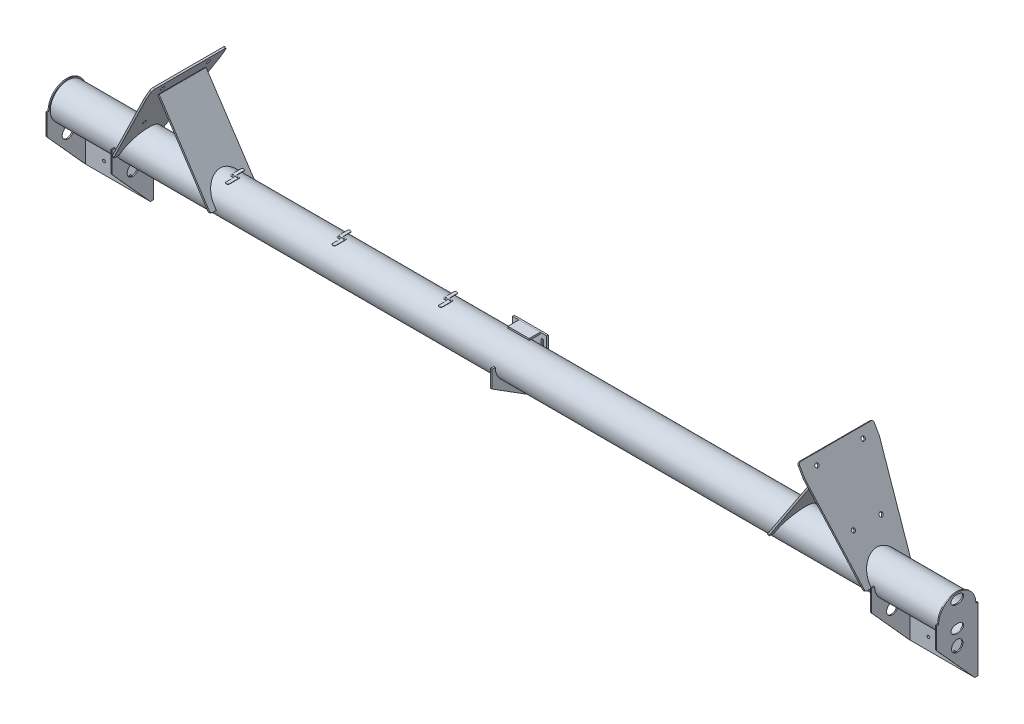
from build123d import *

# Parameters (mm, degrees)
SKETCH1_R             = 82.5
SKETCH1_R_2           = 79.5
BOSS_EXTRUDE1_DEPTH   = 2085
SKETCH2_R             = 26.5
SKETCH2_RX            = 30
SKETCH2_RY            = 20
BOSS_EXTRUDE2_DEPTH   = 5
SKETCH3_R             = 26.5
BOSS_EXTRUDE3_DEPTH   = 5
SKETCH4_W             = 300
SKETCH4_H             = 300
BOSS_EXTRUDE4_DEPTH   = 8
EXTRUDE_THIN1_DEPTH   = 175
EXTRUDE_THIN2_DEPTH   = 110
CUT_EXTRUDE1_DEPTH    = 600
SKETCH19_R            = 9
CUT_EXTRUDE5_DEPTH    = 8
FILLET1_R             = 10
FILLET2_R             = 10
SKETCH7_W             = 160
SKETCH7_H             = 268
BOSS_EXTRUDE5_DEPTH   = 8
BOSS_EXTRUDE6_DEPTH   = 4
SKETCH9_W             = 100
SKETCH9_H             = 52
BOSS_EXTRUDE7_DEPTH   = 8
FILLET3_R             = 10
CUT_EXTRUDE2_DEPTH    = 8
SKETCH17_R            = 6.5
CUT_EXTRUDE3_DEPTH    = 8
SKETCH18_R            = 6.5
CUT_EXTRUDE4_DEPTH    = 8
CUT_EXTRUDE6_DEPTH    = 8
CUT_EXTRUDE7_DEPTH    = 8
BOSS_EXTRUDE8_START   = 82.5
SKETCH22_R            = 3
BOSS_EXTRUDE8_DEPTH   = 1.5
BOSS_EXTRUDE8_2_DEPTH = 1.5
BOSS_EXTRUDE8_3_DEPTH = 1.5


with BuildPart() as part:
    # Sketch1 → Boss-Extrude1 (new, symmetric)
    with BuildSketch(Plane(origin=(0, 0, 0), x_dir=(0, 0, -1), z_dir=(1, 0, 0))):
        Circle(SKETCH1_R)
        Circle(SKETCH1_R_2, mode=Mode.SUBTRACT)
    extrude(amount=BOSS_EXTRUDE1_DEPTH, both=True)


with BuildPart() as body_2:
    # Sketch2 → Boss-Extrude2 (new body)
    with BuildSketch(Plane(origin=(2085, 0, 0), x_dir=(0, 0, -1), z_dir=(1, 0, 0))):
        with BuildLine():
            Line((87.5, 0), (97.5, 0))
            Line((97.5, 0), (97.5, -300))
            Line((97.5, -300), (82.5, -300))
            Line((82.5, -300), (-97.5, -100))
            Line((-97.5, -100), (-97.5, 0))
            Line((-97.5, 0), (-87.5, 0))
            ThreePointArc((-87.5, 0), (0, 87.5), (87.5, 0))
        make_face()
        with Locations((0, -130)):
            Circle(SKETCH2_R, mode=Mode.SUBTRACT)
        with Locations((0, 59.5)):
            Ellipse(SKETCH2_RX, SKETCH2_RY, mode=Mode.SUBTRACT)
        with Locations((0, -59.5)):
            Ellipse(SKETCH2_RX, SKETCH2_RY, mode=Mode.SUBTRACT)
    extrude(amount=BOSS_EXTRUDE2_DEPTH)


with BuildPart() as body_3:
    # Sketch3 → Boss-Extrude3 (new body)
    with BuildSketch(Plane.ZY.offset(-1785)):
        with BuildLine():
            Line((97.5, 0), (97.5, -100))
            Line((97.5, -100), (-82.5, -300))
            Line((-82.5, -300), (-97.5, -300))
            Line((-97.5, -300), (-97.5, 0))
            Line((-97.5, 0), (-82.6, 0))
            ThreePointArc((-82.6, 0), (0, -82.6), (82.6, 0))
            Line((82.6, 0), (97.5, 0))
        make_face()
        with Locations((0, -130)):
            Circle(SKETCH3_R, mode=Mode.SUBTRACT)
    extrude(amount=BOSS_EXTRUDE3_DEPTH)


with BuildPart() as body_4:
    # Sketch4 → Boss-Extrude4 (new body)
    with BuildSketch(Plane(origin=(0, 0, -82.6), x_dir=(-1, 0, 0), z_dir=(0, 0, -1))):
        with Locations((-1935, -150)):
            Rectangle(SKETCH4_W, SKETCH4_H)
    extrude(amount=BOSS_EXTRUDE4_DEPTH)


with BuildPart() as body_5:
    # Sketch 5_3 → Extrude-Thin1 (new, symmetric)
    with BuildSketch(Plane.XY):
        Polygon((1513.109525527, 413.651394229), (1762, -20), (1768.938422308, -16.017752408), (1520.047947835, 417.633641821), align=None)
    extrude(amount=EXTRUDE_THIN1_DEPTH, both=True)


with BuildPart() as body_6:
    # Sketch 5_3 2 → Extrude-Thin2 (new, symmetric)
    with BuildSketch(Plane.XY):
        Polygon((1552.932001443, 344.267171152), (1312, -20), (1305.327470607, -15.58668475), (1546.259472049, 348.680486402), align=None)
    extrude(amount=EXTRUDE_THIN2_DEPTH, both=True)


with BuildPart() as cut_extrude1_tool:
    # Sketch6 → Cut-Extrude1 (new body)
    with BuildSketch(Plane.ZY.offset(-1785)):
        with BuildLine():
            Line((-82.5, 0), (-82.5, -100))
            Line((-82.5, -100), (82.5, -100))
            Line((82.5, -100), (82.5, 0))
            ThreePointArc((82.5, 0), (0, 82.5), (-82.5, 0))
        make_face()
    extrude(amount=CUT_EXTRUDE1_DEPTH)


with BuildPart() as body_6_1:
    add(body_6.part)

    # Cut-Extrude1: cut by cut_extrude1_tool
    add(cut_extrude1_tool.part, mode=Mode.SUBTRACT)

    # Fillet2
    fillet2_edges = [body_6_1.edges().sort_by_distance(p)[0] for p in [
        (1308.663735303, -17.793342375, -110),
        (1308.663735303, -17.793342375, 110),
    ]]
    fillet(fillet2_edges, radius=FILLET2_R)


with BuildPart() as body_5_1:
    add(body_5.part)

    # Cut-Extrude1: cut by cut_extrude1_tool
    add(cut_extrude1_tool.part, mode=Mode.SUBTRACT)

    # Sketch19 → Cut-Extrude5 (cut)
    with BuildSketch(Plane(origin=(1323.705177746, 759.729160648, 0), x_dir=(0, 0, -1), z_dir=(0.8673027884579109, 0.4977809489455502, 0))):
        with Locations(Location((-108.807238687, -434.436087811, 0), (0, 0, 90))):
            Circle(SKETCH19_R)
        with Locations(Location((-65, -690.718989774, 0), (0, 0, 90))):
            Circle(SKETCH19_R)
        with Locations(Location((65, -690.718989774, 0), (0, 0, 90))):
            Circle(SKETCH19_R)
        with Locations(Location((108.807238687, -434.436087811, 0), (0, 0, 90))):
            Circle(SKETCH19_R)
        Polygon((-175, -454.436087811), (-175, -894.436087811), (-110, -894.436087811), align=None)
        Polygon((110, -894.436087811), (175, -454.436087811), (175, -894.436087811), align=None)
    extrude(amount=-CUT_EXTRUDE5_DEPTH, mode=Mode.SUBTRACT)

    # Fillet1
    fillet1_edges = [body_5_1.edges().sort_by_distance(p)[0] for p in [
        (1516.578736681, 415.642518025, 175),
        (1516.578736681, 415.642518025, -175),
        (1765.469211154, -18.008876204, -110),
        (1765.469211154, -18.008876204, 110),
    ]]
    fillet(fillet1_edges, radius=FILLET1_R)


with BuildPart() as body_7:
    # Mirror2: mirrored copy
    add(body_2.part.mirror(Plane(origin=(0, 0, 0), x_dir=(0, 0, 1), z_dir=(1, 0, 0))))


with BuildPart() as body_8:
    # Mirror2 2: mirrored copy
    add(body_4.part.mirror(Plane(origin=(0, 0, 0), x_dir=(0, 0, 1), z_dir=(1, 0, 0))))

    # Sketch18 → Cut-Extrude4 (cut)
    with BuildSketch(Plane.XY.offset(-82.6)):
        with Locations((-1873.483275722, -118.336372909)):
            Circle(SKETCH18_R)
        with Locations((-1997.861792847, -118.336372909)):
            Circle(SKETCH18_R)
        with Locations((-1872.138207153, -244.059958604)):
            Circle(SKETCH18_R)
        with Locations((-1935, -270.098165757)):
            Circle(SKETCH18_R)
        with Locations((-1997.861792847, -244.059958604)):
            Circle(SKETCH18_R)
    extrude(amount=-CUT_EXTRUDE4_DEPTH, mode=Mode.SUBTRACT)

    # Sketch21 → Cut-Extrude7 (cut)
    with BuildSketch(Plane(origin=(0, 0, -90.6), x_dir=(-1, 0, 0), z_dir=(0, 0, -1))):
        with BuildLine():
            Line((2004.361792847, -118.336372909), (2004.361792847, -108.336372909))
            ThreePointArc((2004.361792847, -108.336372909), (1997.861792847, -84.07804266), (1991.361792847, -108.336372909))
            Line((1991.361792847, -108.336372909), (1991.361792847, -118.336372909))
            Line((1991.361792847, -118.336372909), (2004.361792847, -118.336372909))
        make_face()
    extrude(amount=-CUT_EXTRUDE7_DEPTH, mode=Mode.SUBTRACT)


with BuildPart() as body_9:
    # Mirror2 3: mirrored copy
    add(body_3.part.mirror(Plane(origin=(0, 0, 0), x_dir=(0, 0, 1), z_dir=(1, 0, 0))))


with BuildPart() as body_10:
    # Mirror2 4: mirrored copy
    add(body_5_1.part.mirror(Plane(origin=(0, 0, 0), x_dir=(0, 0, 1), z_dir=(1, 0, 0))))


with BuildPart() as body_11:
    # Mirror2 5: mirrored copy
    add(body_6_1.part.mirror(Plane(origin=(0, 0, 0), x_dir=(0, 0, 1), z_dir=(1, 0, 0))))


with BuildPart() as body_12:
    # Sketch7 → Boss-Extrude5 (new body)
    with BuildSketch(Plane(origin=(0, 0, -82.6), x_dir=(-1, 0, 0), z_dir=(0, 0, -1))):
        with Locations((0, -50)):
            Rectangle(SKETCH7_W, SKETCH7_H)
    extrude(amount=BOSS_EXTRUDE5_DEPTH)

    # Fillet3
    fillet3_edges = [body_12.edges().sort_by_distance(p)[0] for p in [
        (-80, -184, -86.6),
        (80, -184, -86.6),
    ]]
    fillet(fillet3_edges, radius=FILLET3_R)

    # Sketch16 → Cut-Extrude2 (cut)
    with BuildSketch(Plane.XY.offset(-82.6)):
        with BuildLine():
            Line((54.65, 26.65), (54.65, 56.65))
            ThreePointArc((54.65, 56.65), (60.15, 62.15), (65.65, 56.65))
            Line((65.65, 56.65), (65.65, 26.65))
            ThreePointArc((65.65, 26.65), (60.15, 21.15), (54.65, 26.65))
        make_face()
        with BuildLine():
            Line((-66, 26.65), (-66, 56.65))
            ThreePointArc((-66, 56.65), (-60.5, 62.15), (-55, 56.65))
            Line((-55, 56.65), (-55, 26.65))
            ThreePointArc((-55, 26.65), (-60.5, 21.15), (-66, 26.65))
        make_face()
        with BuildLine():
            Line((54.65, -157.5), (54.65, -127.5))
            ThreePointArc((54.65, -127.5), (60.15, -122), (65.65, -127.5))
            Line((65.65, -127.5), (65.65, -157.5))
            ThreePointArc((65.65, -157.5), (60.15, -163), (54.65, -157.5))
        make_face()
        with BuildLine():
            Line((-55, -127.5), (-55, -157.5))
            ThreePointArc((-55, -157.5), (-60.5, -163), (-66, -157.5))
            Line((-66, -157.5), (-66, -127.5))
            ThreePointArc((-66, -127.5), (-60.5, -122), (-55, -127.5))
        make_face()
    extrude(amount=-CUT_EXTRUDE2_DEPTH, mode=Mode.SUBTRACT)


with BuildPart() as body_13:
    # Sketch8 → Boss-Extrude6 (new, symmetric)
    with BuildSketch(Plane(origin=(0, 0, 0), x_dir=(0, 0, -1), z_dir=(1, 0, 0))):
        with BuildLine():
            Line((-82.6, 0), (-97.6, 0))
            Line((-97.6, 0), (-97.6, -80))
            Line((-97.6, -80), (67.6, -184))
            Line((67.6, -184), (82.6, -184))
            Line((82.6, -184), (82.6, -34))
            Line((82.6, -34), (75.277885199, -34))
            ThreePointArc((75.277885199, -34), (-17.389748166, -80.748725431), (-82.6, 0))
        make_face()
    extrude(amount=BOSS_EXTRUDE6_DEPTH, both=True)


with BuildPart() as body_14:
    # Sketch9 → Boss-Extrude7 (new body)
    with BuildSketch(Plane(origin=(0, 84, 0), x_dir=(1, 0, 0), z_dir=(0, 1, 0))):
        with Locations((0, 56.6)):
            Rectangle(SKETCH9_W, SKETCH9_H)
    extrude(amount=-BOSS_EXTRUDE7_DEPTH)


with BuildPart() as body_4_1:
    add(body_4.part)

    # Sketch17 → Cut-Extrude3 (cut)
    with BuildSketch(Plane.XY.offset(-82.6)):
        with Locations((1872.138207153, -118.336372909)):
            Circle(SKETCH17_R)
        with Locations((1872.138207153, -244.059958604)):
            Circle(SKETCH17_R)
        with Locations((1935, -270.098165757)):
            Circle(SKETCH17_R)
        with Locations((1997.861792847, -244.059958604)):
            Circle(SKETCH17_R)
        with Locations((1996.516724278, -118.336372909)):
            Circle(SKETCH17_R)
    extrude(amount=-CUT_EXTRUDE3_DEPTH, mode=Mode.SUBTRACT)

    # Sketch20 → Cut-Extrude6 (cut)
    with BuildSketch(Plane(origin=(0, 0, -90.6), x_dir=(-1, 0, 0), z_dir=(0, 0, -1))):
        with BuildLine():
            Line((-1990.016724278, -118.336372909), (-1990.016724278, -108.336372909))
            ThreePointArc((-1990.016724278, -108.336372909), (-1996.516724278, -84.07804266), (-2003.016724278, -108.336372909))
            Line((-2003.016724278, -108.336372909), (-2003.016724278, -118.336372909))
            Line((-2003.016724278, -118.336372909), (-1990.016724278, -118.336372909))
        make_face()
    extrude(amount=-CUT_EXTRUDE6_DEPTH, mode=Mode.SUBTRACT)


with BuildPart() as body_15:
    # Sketch22 → Boss-Extrude8 (new body)
    with BuildSketch(Plane(origin=(0, 0, 0), x_dir=(1, 0, 0), z_dir=(0, 1, 0)).offset(BOSS_EXTRUDE8_START)):
        with BuildLine():
            Line((-1302, 8), (-1288, 8))
            ThreePointArc((-1288, 8), (-1284.464466094, 6.535533906), (-1283, 3))
            Line((-1283, 3), (-1283, -45))
            ThreePointArc((-1283, -45), (-1284.464466094, -48.535533906), (-1288, -50))
            Line((-1288, -50), (-1293, -50))
            ThreePointArc((-1293, -50), (-1296.535533906, -48.535533906), (-1298, -45))
            Line((-1298, -45), (-1298, -8))
            Line((-1298, -8), (-1312, -8))
            ThreePointArc((-1312, -8), (-1315.535533906, -6.535533906), (-1317, -3))
            Line((-1317, -3), (-1317, 45))
            ThreePointArc((-1317, 45), (-1315.535533906, 48.535533906), (-1312, 50))
            Line((-1312, 50), (-1307, 50))
            ThreePointArc((-1307, 50), (-1303.464466094, 48.535533906), (-1302, 45))
            Line((-1302, 45), (-1302, 8))
        make_face()
        with Locations(Location((-1300, 0, 0), (0, 0, 270))):
            Circle(SKETCH22_R, mode=Mode.SUBTRACT)
        with Locations(Location((-1290, 0, 0), (0, 0, 270))):
            Circle(SKETCH22_R, mode=Mode.SUBTRACT)
        with Locations(Location((-1310, 0, 0), (0, 0, 270))):
            Circle(SKETCH22_R, mode=Mode.SUBTRACT)
    extrude(amount=BOSS_EXTRUDE8_DEPTH)


with BuildPart() as body_16:
    # Sketch22 → Boss-Extrude8 2 (new body)
    with BuildSketch(Plane(origin=(0, 0, 0), x_dir=(1, 0, 0), z_dir=(0, 1, 0)).offset(BOSS_EXTRUDE8_START)):
        with BuildLine():
            Line((-302, 8), (-288, 8))
            ThreePointArc((-288, 8), (-284.464466094, 6.535533906), (-283, 3))
            Line((-283, 3), (-283, -45))
            ThreePointArc((-283, -45), (-284.464466094, -48.535533906), (-288, -50))
            Line((-288, -50), (-293, -50))
            ThreePointArc((-293, -50), (-296.535533906, -48.535533906), (-298, -45))
            Line((-298, -45), (-298, -8))
            Line((-298, -8), (-312, -8))
            ThreePointArc((-312, -8), (-315.535533906, -6.535533906), (-317, -3))
            Line((-317, -3), (-317, 45))
            ThreePointArc((-317, 45), (-315.535533906, 48.535533906), (-312, 50))
            Line((-312, 50), (-307, 50))
            ThreePointArc((-307, 50), (-303.464466094, 48.535533906), (-302, 45))
            Line((-302, 45), (-302, 8))
        make_face()
        with Locations(Location((-300, 0, 0), (0, 0, 270))):
            Circle(SKETCH22_R, mode=Mode.SUBTRACT)
        with Locations(Location((-290, 0, 0), (0, 0, 270))):
            Circle(SKETCH22_R, mode=Mode.SUBTRACT)
        with Locations(Location((-310, 0, 0), (0, 0, 270))):
            Circle(SKETCH22_R, mode=Mode.SUBTRACT)
    extrude(amount=BOSS_EXTRUDE8_2_DEPTH)


with BuildPart() as body_17:
    # Sketch22 → Boss-Extrude8 3 (new body)
    with BuildSketch(Plane(origin=(0, 0, 0), x_dir=(1, 0, 0), z_dir=(0, 1, 0)).offset(BOSS_EXTRUDE8_START)):
        with BuildLine():
            Line((-802, 8), (-788, 8))
            ThreePointArc((-788, 8), (-784.464466094, 6.535533906), (-783, 3))
            Line((-783, 3), (-783, -45))
            ThreePointArc((-783, -45), (-784.464466094, -48.535533906), (-788, -50))
            Line((-788, -50), (-793, -50))
            ThreePointArc((-793, -50), (-796.535533906, -48.535533906), (-798, -45))
            Line((-798, -45), (-798, -8))
            Line((-798, -8), (-812, -8))
            ThreePointArc((-812, -8), (-815.535533906, -6.535533906), (-817, -3))
            Line((-817, -3), (-817, 45))
            ThreePointArc((-817, 45), (-815.535533906, 48.535533906), (-812, 50))
            Line((-812, 50), (-807, 50))
            ThreePointArc((-807, 50), (-803.464466094, 48.535533906), (-802, 45))
            Line((-802, 45), (-802, 8))
        make_face()
        with Locations(Location((-800, 0, 0), (0, 0, 270))):
            Circle(SKETCH22_R, mode=Mode.SUBTRACT)
        with Locations(Location((-790, 0, 0), (0, 0, 270))):
            Circle(SKETCH22_R, mode=Mode.SUBTRACT)
        with Locations(Location((-810, 0, 0), (0, 0, 270))):
            Circle(SKETCH22_R, mode=Mode.SUBTRACT)
    extrude(amount=BOSS_EXTRUDE8_3_DEPTH)


solid = Compound([part.part, body_2.part, body_3.part, body_6_1.part, body_5_1.part, body_7.part, body_8.part, body_9.part, body_10.part, body_11.part, body_12.part, body_13.part, body_14.part, body_4_1.part, body_15.part, body_16.part, body_17.part])
